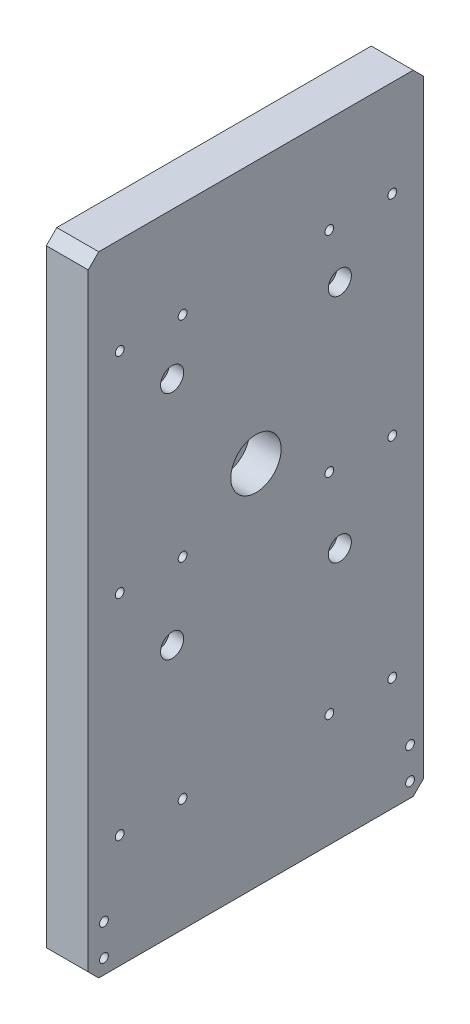
SolidWorks part; units mm, degrees
material "A6061 T6"
ref_plane "前视基准面" through (0, 0, 0) normal (0, 0, 1) x (1, 0, 0)
ref_plane "上视基准面" through (0, 0, 0) normal (0, 1, 0) x (1, 0, 0)
ref_plane "右视基准面" through (0, 0, 0) normal (1, 0, 0) x (0, 0, -1)
sketch "草图1" plane through (0, 0, 0) normal (1, 0, 0) x (0, 0, -1)
  line L1 (-80, 150) -> (80, 150)
  line L2 (-80, 150) -> (-80, -150)
  line L3 (-80, -150) -> (80, -150)
  line L4 (80, 150) -> (80, -150)
  line L5 (-80, 150) -> (80, -150) construction
  line L6 (-80, -150) -> (80, 150) construction
  point P0 (0, 0)
  dimension "D1" = 160
  dimension "D2" = 300
extrude "凸台-拉伸1" add sketch "草图1" along normal blind 20
hole_wizard "打孔尺寸(%根据)内六角圆柱头螺钉的类型1" positions "草图2" profile "草图3" counterbore size "M14" standard "GB"
sketch "草图2" plane through (20, 0, 0) normal (1, 0, 0) x (0, 0, -1)
  line L0 (80, 150) -> (-80, 150) construction
  point P0 (0, 25)
  dimension "D1" = 125
sketch "草图3" plane through (20, 25, 0) normal (0, 1, 0) x (0, 0, -1)
  line L0 (0, 0) -> (0, 29.6567)
  line L1 (0, 29.6567) -> (7.75, 25)
  line L2 (7.75, 25) -> (7.75, 15)
  line L3 (7.75, 15) -> (12, 15)
  line L4 (12, 15) -> (12, 0)
  line L5 (12, 0) -> (0, 0)
  line L10 (0, 29.6567) -> (-7.75, 25) construction
  line L11 (0, -6.35) -> (0, 107.95) construction
  dimension "孔直径" = 15.5
  dimension "孔深度" = 25
  dimension "柱形沉头孔直径" = 24
  dimension "柱形沉头孔深度" = 15
  dimension "导头角度" = 118
chamfer "倒角1" distance 5 angle 45 4 edges at (10, 150, 80) (10, 150, -80) (10, -150, -80) (10, -150, 80)
hole_wizard "打孔尺寸(%根据)内六角圆柱头螺钉的类型0" positions "草图4" profile "草图5" counterbore size "M6" standard "GB"
sketch "草图4" plane through (20, 0, 0) normal (1, 0, 0) x (0, 0, -1)
  point P0 (40, -30)
  point P2 (40, 80)
  point P16 (-40, -30)
  point P19 (-40, 80)
sketch "草图5" plane through (20, -30, -40) normal (0, 1, 0) x (0, 0, -1)
  line L0 (0, 0) -> (0, 26.9828)
  line L1 (0, 26.9828) -> (3.3, 25)
  line L2 (3.3, 25) -> (3.3, 6.8)
  line L3 (3.3, 6.8) -> (5.5, 6.8)
  line L4 (5.5, 6.8) -> (5.5, 0)
  line L5 (5.5, 0) -> (0, 0)
  line L10 (0, 26.9828) -> (-3.3, 25) construction
  line L11 (0, -6.35) -> (0, 107.95) construction
  dimension "孔直径" = 6.6
  dimension "孔深度" = 25
  dimension "柱形沉头孔直径" = 11
  dimension "柱形沉头孔深度" = 6.8
  dimension "导头角度" = 118
sketch "草图6" plane through (0, 0, 0) normal (-1, 0, 0) x (0, 0, 1)
  circle A0 centre (-40, 80) radius 8.1
  circle A1 centre (-40, -30) radius 8.1
  circle A2 centre (0, 25) radius 10
  circle A3 centre (40, -30) radius 8.1
  circle A4 centre (40, 80) radius 8.1
  dimension "D1" = 16.2
  dimension "D2" = 20
  dimension "D3" = 16.2
extrude "切除-拉伸1" cut sketch "草图6" against normal blind 2
hole_wizard "M5 螺纹孔1" positions "草图7" profile "草图8" tap size "M5" standard "GB"
sketch "草图7" plane through (0, 0, 0) normal (-1, 0, 0) x (0, 0, 1)
  point P0 (65, -96)
  point P3 (35, -96)
  point P6 (65, 4)
  point P9 (35, 4)
  point P12 (65, 104)
  point P15 (35, 104)
  point P18 (-35, 104)
  point P21 (-65, 104)
  point P24 (-35, 4)
  point P27 (-65, 4)
  point P30 (-35, -96)
  point P33 (-65, -96)
sketch "草图8" plane through (0, -96, 65) normal (0, 1, 0) x (0, 0, 1)
  line L0 (0, 0) -> (0, 21.2618)
  line L1 (0, 21.2618) -> (2.1, 20)
  line L2 (2.1, 20) -> (2.1, 0)
  line L5 (2.1, 0) -> (0, 0)
  line L10 (0, 21.2618) -> (-2.1, 20) construction
  line L11 (0, -6.35) -> (0, 107.95) construction
  dimension "螺纹孔钻头直径" = 4.2
  dimension "螺纹孔钻头深度" = 20
  dimension "导头角度" = 118
cosmetic thread "孔螺蚊线1"
cosmetic thread "孔螺蚊线2"
cosmetic thread "孔螺蚊线3"
cosmetic thread "孔螺蚊线4"
cosmetic thread "孔螺蚊线5"
cosmetic thread "孔螺蚊线6"
cosmetic thread "孔螺蚊线9"
cosmetic thread "孔螺蚊线10"
cosmetic thread "孔螺蚊线11"
cosmetic thread "孔螺蚊线12"
cosmetic thread "孔螺蚊线17"
cosmetic thread "孔螺蚊线18"
hole_wizard "M5 螺纹孔2" positions "草图9" profile "草图10" tap size "M5" standard "GB"
sketch "草图9" plane through (0, 0, 0) normal (-1, 0, 0) x (0, 0, 1)
  point P0 (72.5, -143)
  point P3 (72.5, -128)
sketch "草图10" plane through (0, -143, 72.5) normal (0, 1, 0) x (0, 0, 1)
  line L0 (0, 0) -> (0, 21.2618)
  line L1 (0, 21.2618) -> (2.1, 20)
  line L2 (2.1, 20) -> (2.1, 0)
  line L5 (2.1, 0) -> (0, 0)
  line L10 (0, 21.2618) -> (-2.1, 20) construction
  line L11 (0, -6.35) -> (0, 107.95) construction
  dimension "螺纹孔钻头直径" = 4.2
  dimension "螺纹孔钻头深度" = 20
  dimension "导头角度" = 118
cosmetic thread "孔螺蚊线13"
cosmetic thread "孔螺蚊线14"
hole_wizard "M5 螺纹孔3" positions "草图11" profile "草图12" tap size "M5" standard "GB"
sketch "草图11" plane through (0, 0, 0) normal (-1, 0, 0) x (0, 0, 1)
  point P0 (-73.5, -143)
  point P3 (-73.5, -128)
sketch "草图12" plane through (0, -143, -73.5) normal (0, 1, 0) x (0, 0, 1)
  line L0 (0, 0) -> (0, 26.2618)
  line L1 (0, 26.2618) -> (2.1, 25)
  line L2 (2.1, 25) -> (2.1, 0)
  line L5 (2.1, 0) -> (0, 0)
  line L10 (0, 26.2618) -> (-2.1, 25) construction
  line L11 (0, -6.35) -> (0, 107.95) construction
  dimension "螺纹孔钻头直径" = 4.2
  dimension "螺纹孔钻头深度" = 25
  dimension "导头角度" = 118
cosmetic thread "孔螺蚊线15"
cosmetic thread "孔螺蚊线16"
